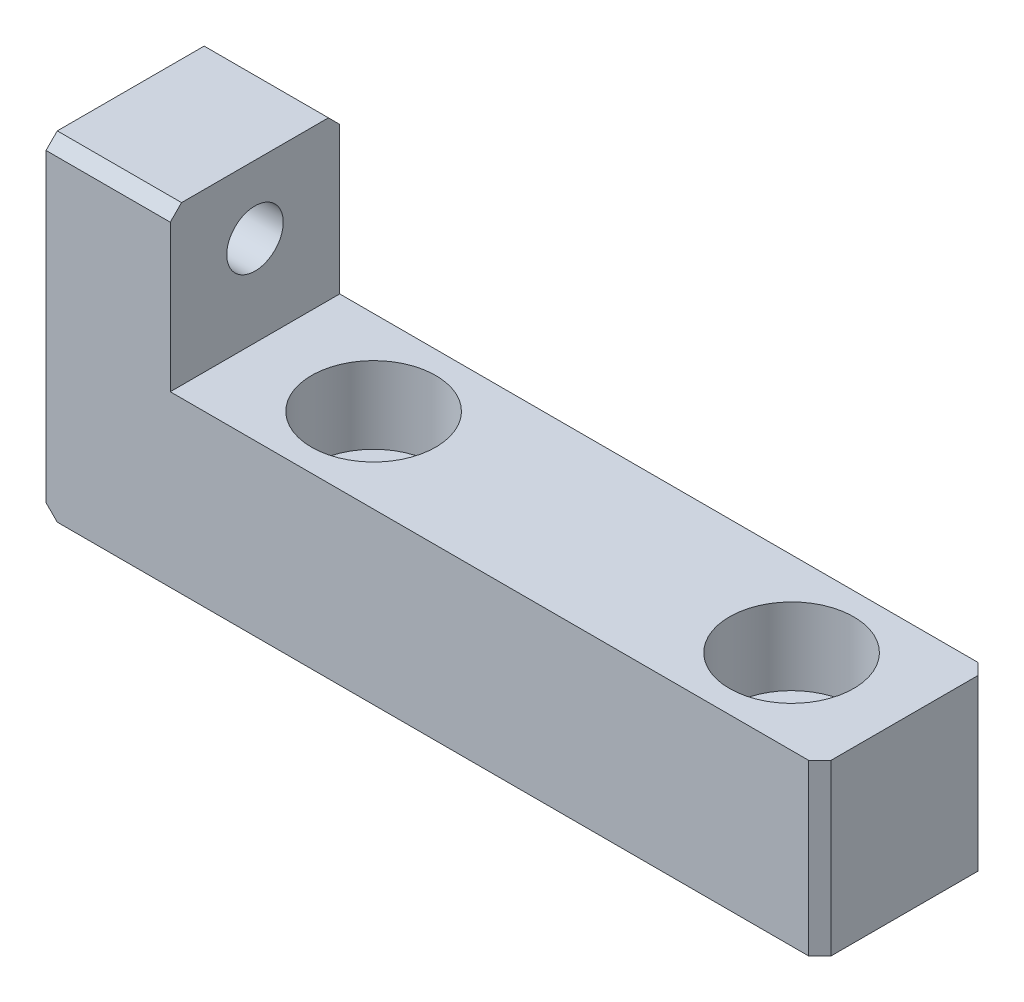
from build123d import *

# Parameters (mm, degrees)
SKETCH_1_W                   = 68.5
SKETCH_1_H                   = 15
EXTRUDE_1_DEPTH              = 7.5
SKETCH_2_W                   = 11
SKETCH_2_H                   = 15
EXTRUDE_2_DEPTH              = 14
CHAMFER_1_SIZE               = 1
HOLE_WIZARD_M6_1_D           = 6.6
HOLE_WIZARD_M6_1_CBORE_D     = 11
HOLE_WIZARD_M6_1_CBORE_DEPTH = 6.8
HOLE_WIZARD_M6_1_2_D         = 5


with BuildPart() as part:
    # 草图1 → 凸台-拉伸1 (new, symmetric)
    with BuildSketch(Plane(origin=(0, 0, 0), x_dir=(1, 0, 0), z_dir=(0, 1, 0))):
        Rectangle(SKETCH_1_W, SKETCH_1_H)
    extrude(amount=EXTRUDE_1_DEPTH, both=True)

    # 草图2 → 凸台-拉伸2 (add)
    with BuildSketch(Plane(origin=(0, 7.5, 0), x_dir=(1, 0, 0), z_dir=(0, 1, 0))):
        with Locations((-28.75, 0)):
            Rectangle(SKETCH_2_W, SKETCH_2_H)
    extrude(amount=EXTRUDE_2_DEPTH)

    # 倒角1
    chamfer_1_edges = [part.edges().sort_by_distance(p)[0] for p in [
        (-28.75, 21.5, 7.5),
        (-28.75, 21.5, -7.5),
        (-34.25, -7.5, 0),
        (34.25, 0, 7.5),
        (34.25, 0, -7.5),
    ]]
    chamfer(chamfer_1_edges, length=CHAMFER_1_SIZE)

    # Hole Wizard M6 _1 (through all)
    with Locations(Plane(origin=(0, 7.5, 0), x_dir=(1, 0, 0), z_dir=(0, 1, 0))):
        with Locations((24.25, 0), (-12.75, 0)):
            CounterBoreHole(HOLE_WIZARD_M6_1_D / 2, HOLE_WIZARD_M6_1_CBORE_D / 2, HOLE_WIZARD_M6_1_CBORE_DEPTH)

    # Hole Wizard M6 _1 2 (through all)
    with Locations(Plane.ZY.offset(34.25)):
        with Locations((0, 15.5)):
            Hole(HOLE_WIZARD_M6_1_2_D / 2)


solid = part.part
